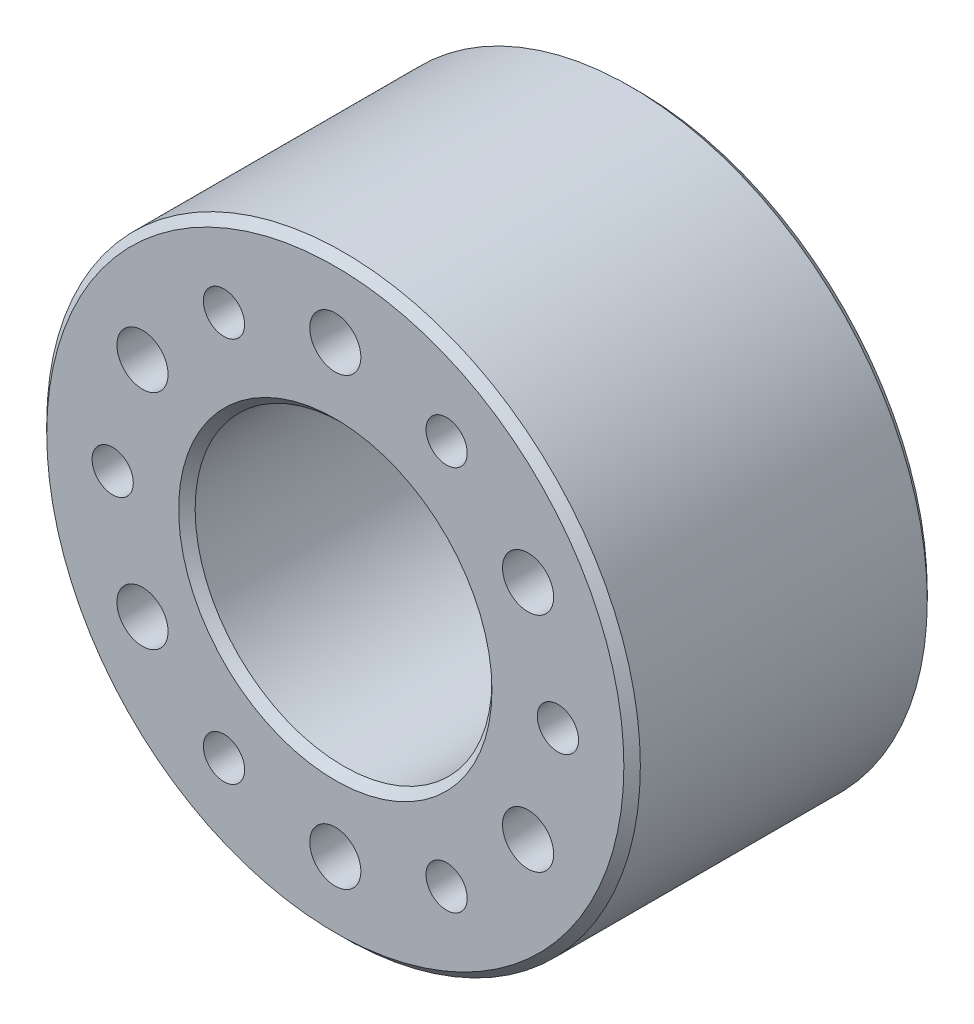
SolidWorks part; units mm, degrees
material "6061 合金"
ref_plane "前视基准面" through (0, 0, 0) normal (0, 0, 1) x (1, 0, 0)
ref_plane "上视基准面" through (0, 0, 0) normal (0, 1, 0) x (1, 0, 0)
ref_plane "右视基准面" through (0, 0, 0) normal (1, 0, 0) x (0, 0, -1)
other "Configuration Table"
sketch "草图1" plane through (0, 0, 0) normal (0, 0, 1) x (1, 0, 0)
  circle A0 centre (0, 0) radius 13.5 construction
  circle A1 centre (0, 13.5) radius 1.55
  circle A2 centre (11.6913, 6.75) radius 1.55
  circle A3 centre (11.6913, -6.75) radius 1.55
  circle A4 centre (0, -13.5) radius 1.55
  circle A5 centre (-11.6913, -6.75) radius 1.55
  circle A6 centre (-11.6913, 6.75) radius 1.55
  circle A7 centre (0, 0) radius 9
  circle A8 centre (0, 0) radius 18
  circle A9 centre (13.5, 0) radius 1.6 construction
  circle A10 centre (6.75, -11.6913) radius 1.6 construction
  circle A11 centre (-6.75, -11.6913) radius 1.6 construction
  circle A12 centre (-13.5, 0) radius 1.6 construction
  circle A13 centre (-6.75, 11.6913) radius 1.6 construction
  circle A14 centre (6.75, 11.6913) radius 1.6 construction
  point P17 (0, 0)
  point P32 (0, 0)
  dimension "D1" = 27
  dimension "D3" = 3.1
  dimension "D4" = 18
  dimension "D5" = 36
  dimension "D6" = 6
  dimension "D7" = 3.2
  dimension "D2" = 6
extrude "凸台-拉伸1" add sketch "草图1" along normal blind 18.4
sketch "草图4" plane through (0, 0, 0) normal (0, 0, 1) x (1, 0, 0)
  circle A0 centre (0, 13.5) radius 3.5
  circle A1 centre (11.6913, 6.75) radius 3.5
  circle A2 centre (11.6913, -6.75) radius 3.5
  circle A3 centre (0, -13.5) radius 3.5
  circle A4 centre (-11.6913, -6.75) radius 3.5
  circle A5 centre (-11.6913, 6.75) radius 3.5
  point P15 (0, 0)
  point P36 (0, 0)
  dimension "D1" = 7
  dimension "D2" = 6
extrude "切除-拉伸1" cut sketch "草图4" along normal blind 7
sketch "草图5" plane through (0, 0, 0) normal (0, 0, -1) x (-1, 0, 0)
  circle A0 centre (0, 0) radius 9
  circle A1 centre (0, 0) radius 10
  circle A2 centre (0, 0) radius 9 construction
  dimension "D1" = 1
extrude "凸台-拉伸2" add sketch "草图5" along normal blind 4
hole_wizard "M3 螺纹孔1" positions "草图2" profile "草图3" tap size "M3" standard "GB" end condition through all
sketch "草图2" plane through (0, 0, 18.4) normal (0, 0, 1) x (1, 0, 0)
  point P0 (13.5, 0)
  point P3 (6.75, -11.6913)
  point P6 (-6.75, -11.6913)
  point P9 (-13.5, 0)
  point P12 (-6.75, 11.6913)
  point P15 (6.75, 11.6913)
cosmetic thread "孔螺蚊线1" parameters "D2"=3
cosmetic thread "孔螺蚊线2" parameters "D2"=3
cosmetic thread "孔螺蚊线3" parameters "D2"=3
cosmetic thread "孔螺蚊线4" parameters "D2"=3
cosmetic thread "孔螺蚊线5" parameters "D2"=3
cosmetic thread "孔螺蚊线6" parameters "D2"=3
sketch "草图3" plane through (13.5, 0, 18.4) normal (1, 0, 0) x (0, -1, 0)
  line L0 (0, 0) -> (0, 22.4)
  line L1 (0, 22.4) -> (1.25, 22.4)
  line L2 (1.25, 22.4) -> (1.25, 0)
  line L5 (1.25, 0) -> (0, 0)
  line L11 (0, -6.35) -> (0, 107.95) construction
  dimension "通孔螺纹孔钻头直径" = 2.5
  dimension "通孔螺纹孔钻头深度" = 22.4
chamfer "倒角1" distance 0.5 angle 45 4 edges at (9, 0, 18.4) (18, 0, 18.4) (18, 0, 0) (-10, 0, -4)
